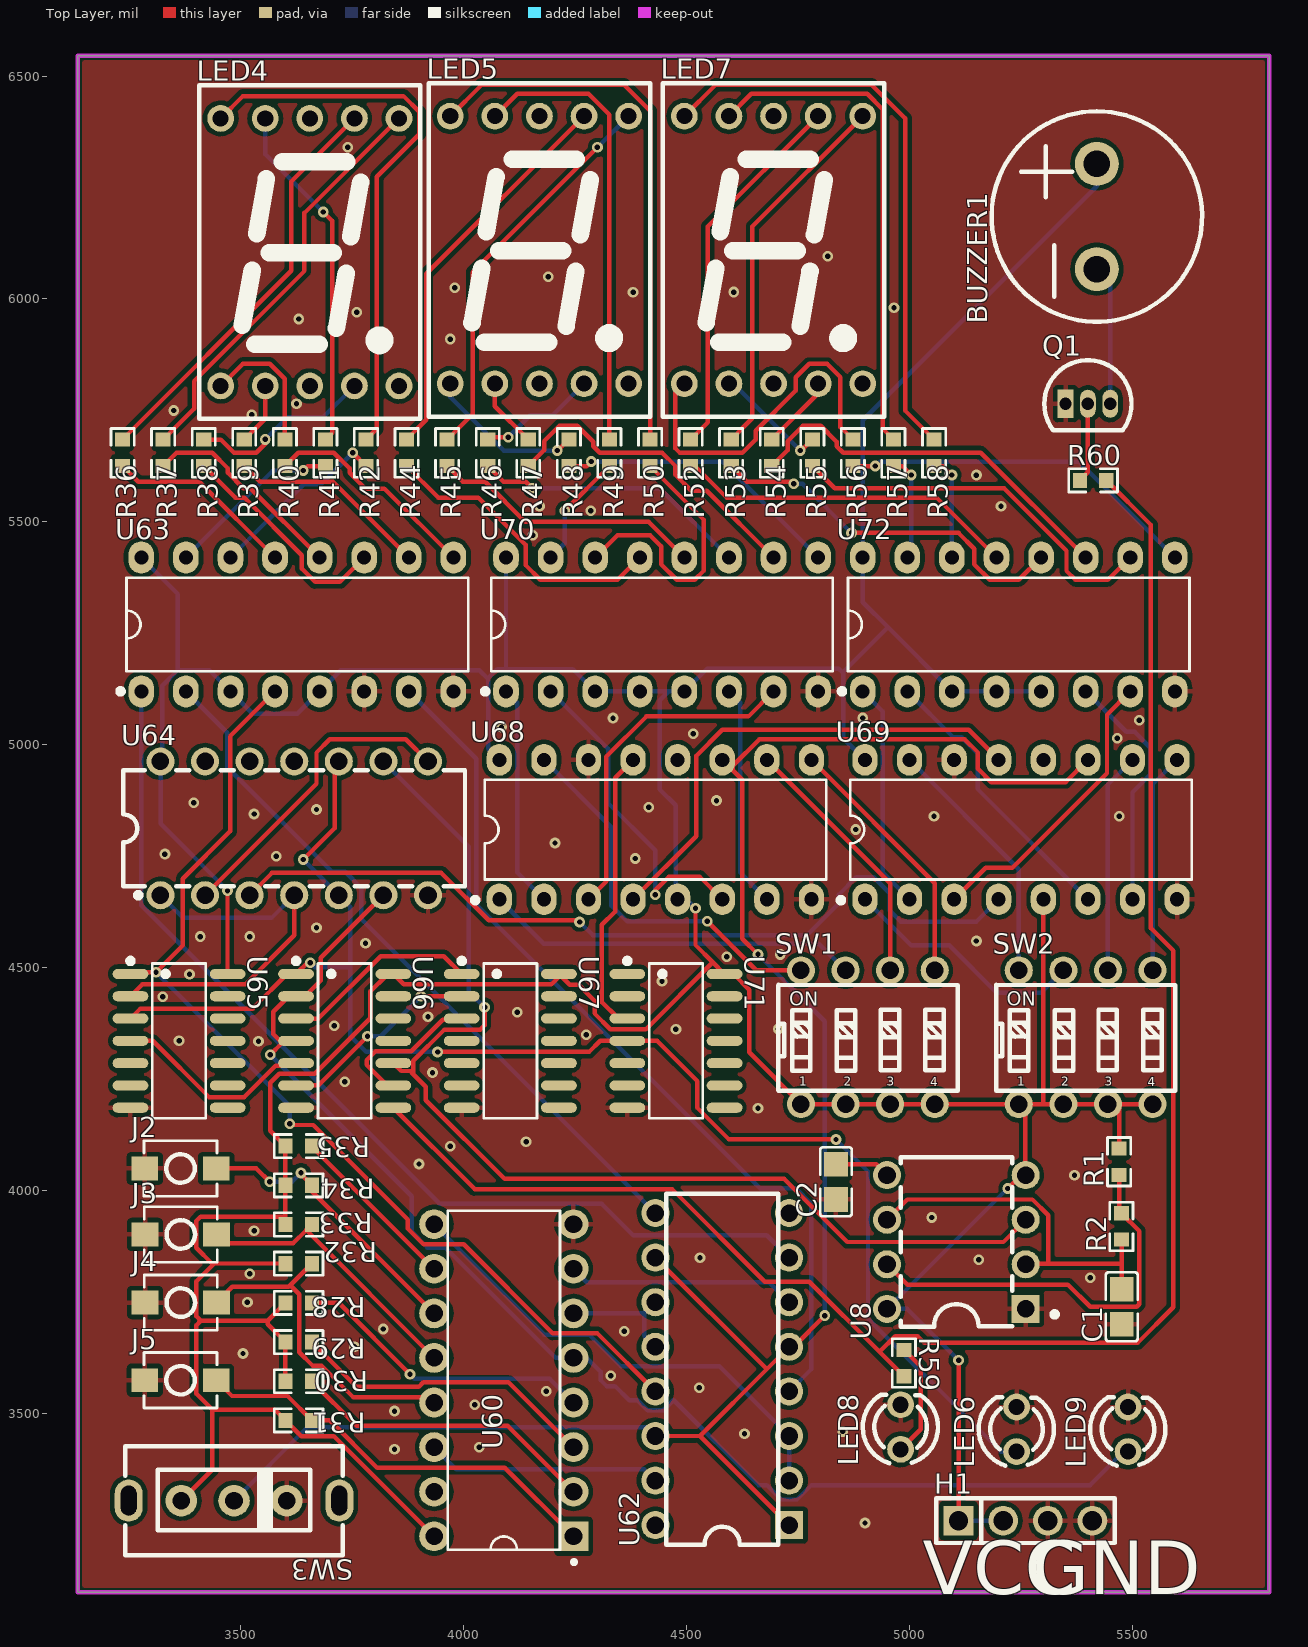
[diagram p0: Top Layer view]
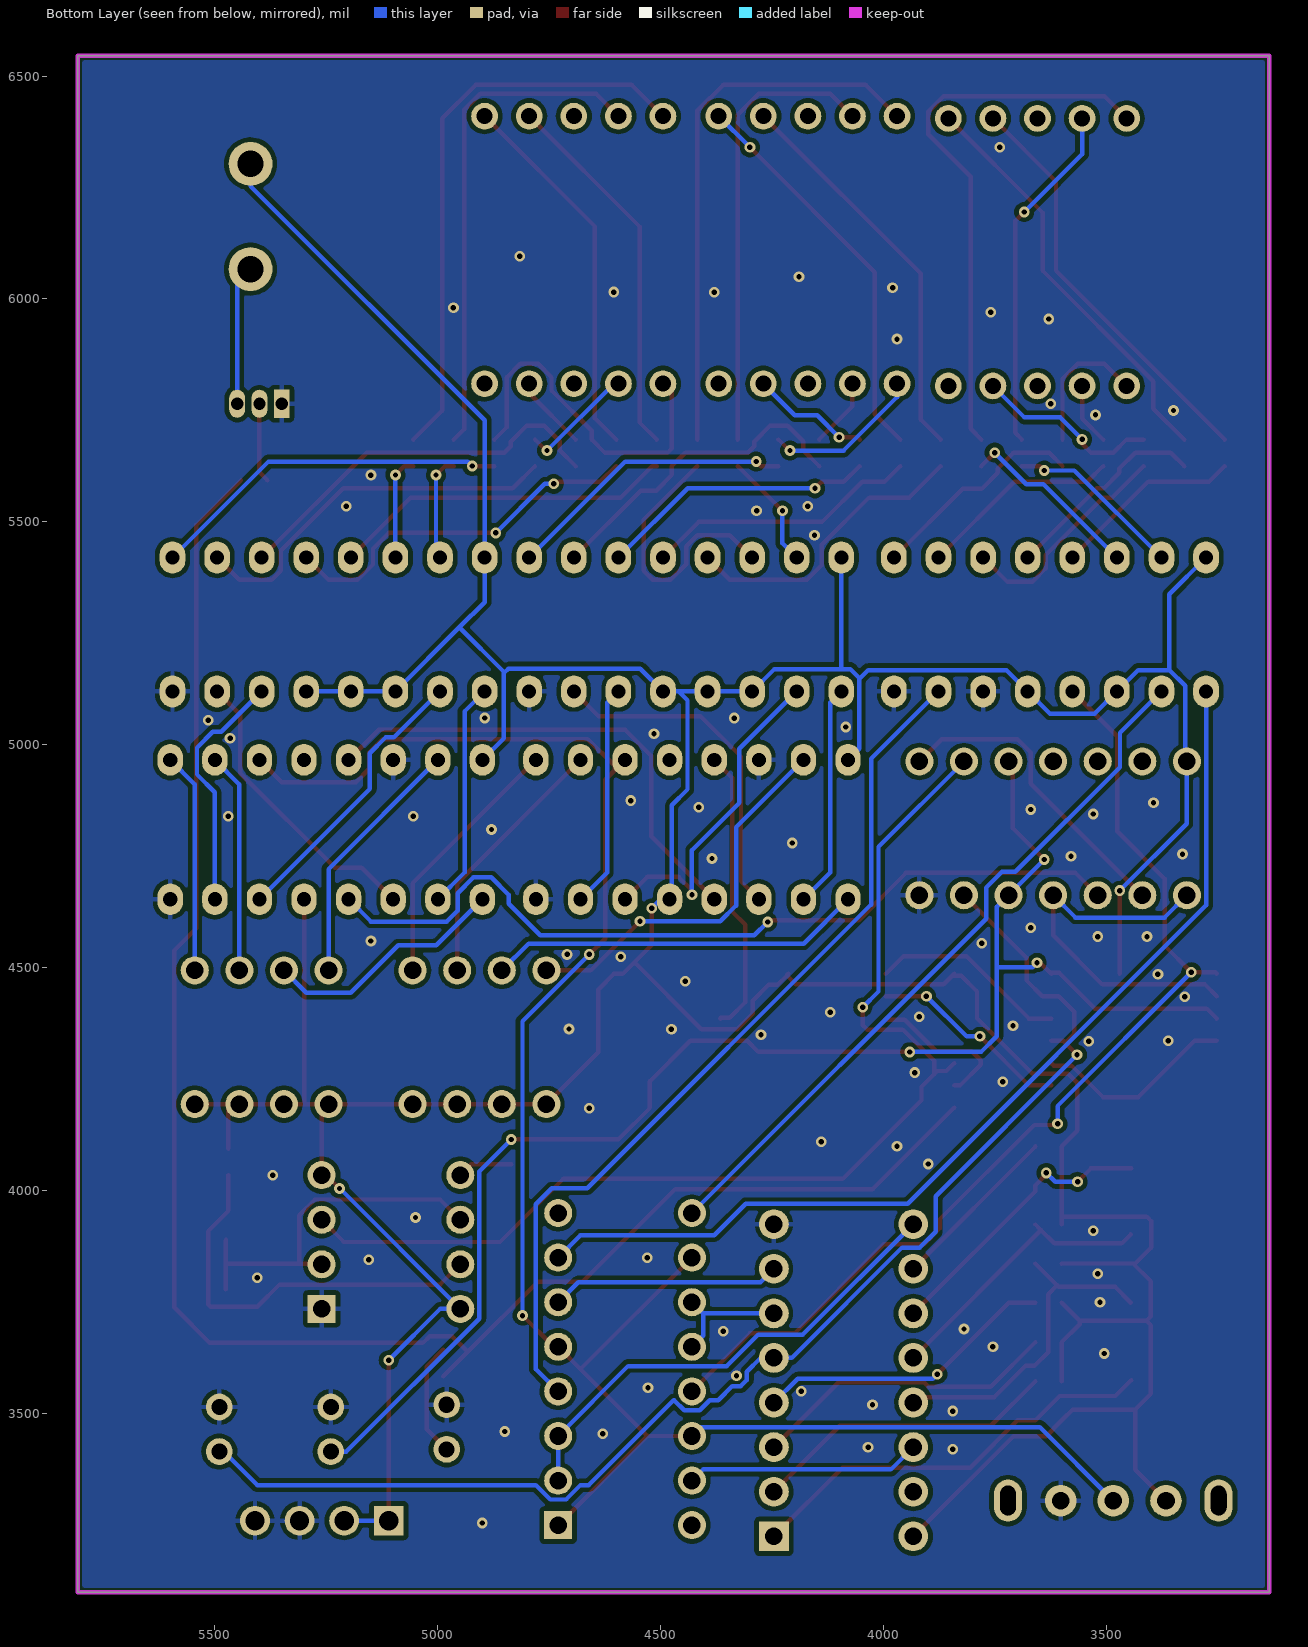
[diagram p1: Bottom Layer view, seen from below]
# Altium PCB MISC75092.pcbdoc
Units mil, origin at the board's own origin, x right, y up, seen from the top; angles counter-clockwise.
Board outline 2672.01 x 3445 mil, 2 copper layers (Top Layer, Bottom Layer), stack 62.206 mil thick; 64 components, 96 nets, 334 pads, 120 vias.

## Layer stack, top to bottom
Top Solder Mask Layer: solder mask 0.394, Dk 3.3
Top Layer: signal copper 1.379
Dielectric1: surface 59.449, FR4, Dk 4.5
Bottom Layer: signal copper 1.378
Bottom Solder Mask Layer: solder mask 0.394, Dk 3.3

## Board outline
3135,6545 3135,3100 5807.01,3100 5807.01,6545

## Design rules (kind name [scope] priority, off if disabled: settings)
BoardOutlineClearance copperThickness2oz_1 [All] p2 off: genericclearance=7.99 ignorepadtopadclearanceinfootprint=FALSE except(0: Arc-SplitContinuation Track-SplitContinuation SMDPad-SplitContinuation THPad-SplitContinuation Via-SplitContinuation Fill-SplitContinuation Region-SplitContinuation Poly-SplitContinuation Text-SplitContinuation Hole-SplitContinuation; 5.98: Arc-CutoutEdge Track-CutoutEdge SMDPad-CutoutEdge THPad-CutoutEdge Via-CutoutEdge Text-CutoutEdge; 6.9: Hole-OutlineEdge Hole-CutoutEdge; 10: Poly-OutlineEdge Poly-CutoutEdge; 11.81: Arc-OutlineEdge Track-OutlineEdge SMDPad-OutlineEdge THPad-OutlineEdge Via-OutlineEdge Fill-OutlineEdge Region-OutlineEdge Text-OutlineEdge Fill-CutoutEdge Region-CutoutEdge)
BoardOutlineClearance Plane_innerPlane_1 [All] p4 off: genericclearance=4.02 ignorepadtopadclearanceinfootprint=FALSE except(0: Arc-SplitContinuation Track-SplitContinuation SMDPad-SplitContinuation THPad-SplitContinuation Via-SplitContinuation Fill-SplitContinuation Region-SplitContinuation Poly-SplitContinuation Text-SplitContinuation Hole-SplitContinuation; 5.98: Arc-CutoutEdge Track-CutoutEdge SMDPad-CutoutEdge THPad-CutoutEdge Via-CutoutEdge Text-CutoutEdge; 6.9: Hole-OutlineEdge Hole-CutoutEdge; 10: Poly-OutlineEdge Poly-CutoutEdge; 11.81: Arc-OutlineEdge Track-OutlineEdge SMDPad-OutlineEdge THPad-OutlineEdge Via-OutlineEdge Fill-OutlineEdge Region-OutlineEdge Text-OutlineEdge Fill-CutoutEdge Region-CutoutEdge)
BoardOutlineClearance Copper_copperRegion_1 [All] p6 off: genericclearance=4.02 ignorepadtopadclearanceinfootprint=FALSE except(0: Arc-SplitContinuation Track-SplitContinuation SMDPad-SplitContinuation THPad-SplitContinuation Via-SplitContinuation Fill-SplitContinuation Region-SplitContinuation Poly-SplitContinuation Text-SplitContinuation Hole-SplitContinuation; 5.98: Arc-CutoutEdge Track-CutoutEdge SMDPad-CutoutEdge THPad-CutoutEdge Via-CutoutEdge Text-CutoutEdge; 6.9: Hole-OutlineEdge Hole-CutoutEdge; 10: Poly-OutlineEdge Poly-CutoutEdge; 11.81: Arc-OutlineEdge Track-OutlineEdge SMDPad-OutlineEdge THPad-OutlineEdge Via-OutlineEdge Fill-OutlineEdge Region-OutlineEdge Text-OutlineEdge Fill-CutoutEdge Region-CutoutEdge)
BoardOutlineClearance copperThickness1oz_1 [All] p8: genericclearance=4.02 ignorepadtopadclearanceinfootprint=FALSE except(0: Arc-SplitContinuation Track-SplitContinuation SMDPad-SplitContinuation THPad-SplitContinuation Via-SplitContinuation Fill-SplitContinuation Region-SplitContinuation Poly-SplitContinuation Text-SplitContinuation Hole-SplitContinuation; 5.98: Arc-CutoutEdge Track-CutoutEdge SMDPad-CutoutEdge THPad-CutoutEdge Via-CutoutEdge Text-CutoutEdge; 6.9: Hole-OutlineEdge Hole-CutoutEdge; 10: Poly-OutlineEdge Poly-CutoutEdge; 11.81: Arc-OutlineEdge Track-OutlineEdge SMDPad-OutlineEdge THPad-OutlineEdge Via-OutlineEdge Fill-OutlineEdge Region-OutlineEdge Text-OutlineEdge Fill-CutoutEdge Region-CutoutEdge)
Clearance copperThickness2oz [All] p1 off: gap=7.99 ignorepadtopadclearanceinfootprint=FALSE except(5.98: SMDPad-Track SMDPad-SMDPad THPad-Track SMDPad-THPad THPad-THPad Track-Via SMDPad-Via THPad-Via Via-Via Fill-SMDPad Region-SMDPad Fill-THPad Region-THPad Fill-Via Region-Via Fill-Fill Fill-Region Region-Region Arc-Track Arc-SMDPad Arc-THPad Arc-Via Fill-Arc Region-Arc Arc-Arc Text-Track SMDPad-Text Text-THPad Text-Via Fill-Text Region-Text Arc-Text Text-Text; 6.9: Hole-Track Hole-SMDPad Hole-THPad Hole-Via Fill-Hole Region-Hole Hole-Arc Hole-Text; 10: Poly-Track Poly-SMDPad Poly-THPad Poly-Via Poly-Fill Poly-Region Poly-Poly Poly-Arc Poly-Text Poly-Hole; 11.81: Fill-Track Region-Track)
Clearance Plane_innerPlane [All] p3 off: gap=4.02 ignorepadtopadclearanceinfootprint=FALSE except(5.98: SMDPad-Track SMDPad-SMDPad THPad-Track SMDPad-THPad THPad-THPad Track-Via SMDPad-Via THPad-Via Via-Via Fill-SMDPad Region-SMDPad Fill-THPad Region-THPad Fill-Via Region-Via Fill-Fill Fill-Region Region-Region Arc-Track Arc-SMDPad Arc-THPad Arc-Via Fill-Arc Region-Arc Arc-Arc Text-Track SMDPad-Text Text-THPad Text-Via Fill-Text Region-Text Arc-Text Text-Text; 6.9: Hole-Track Hole-SMDPad Hole-THPad Hole-Via Fill-Hole Region-Hole Hole-Arc Hole-Text; 10: Poly-Track Poly-SMDPad Poly-THPad Poly-Via Poly-Fill Poly-Region Poly-Poly Poly-Arc Poly-Text Poly-Hole; 11.81: Fill-Track Region-Track)
Clearance Copper_copperRegion [All] p5 off: gap=4.02 ignorepadtopadclearanceinfootprint=FALSE except(5.98: SMDPad-Track SMDPad-SMDPad THPad-Track SMDPad-THPad THPad-THPad Track-Via SMDPad-Via THPad-Via Via-Via Fill-SMDPad Region-SMDPad Fill-THPad Region-THPad Fill-Via Region-Via Fill-Fill Fill-Region Region-Region Arc-Track Arc-SMDPad Arc-THPad Arc-Via Fill-Arc Region-Arc Arc-Arc Text-Track SMDPad-Text Text-THPad Text-Via Fill-Text Region-Text Arc-Text Text-Text; 6.9: Hole-Track Hole-SMDPad Hole-THPad Hole-Via Fill-Hole Region-Hole Hole-Arc Hole-Text; 10: Poly-Track Poly-SMDPad Poly-THPad Poly-Via Poly-Fill Poly-Region Poly-Poly Poly-Arc Poly-Text Poly-Hole; 11.81: Fill-Track Region-Track)
Clearance copperThickness1oz [All] p7: gap=4.02 ignorepadtopadclearanceinfootprint=FALSE except(5.98: SMDPad-Track SMDPad-SMDPad THPad-Track SMDPad-THPad THPad-THPad Track-Via SMDPad-Via THPad-Via Via-Via Fill-SMDPad Region-SMDPad Fill-THPad Region-THPad Fill-Via Region-Via Fill-Fill Fill-Region Region-Region Arc-Track Arc-SMDPad Arc-THPad Arc-Via Fill-Arc Region-Arc Arc-Arc Text-Track SMDPad-Text Text-THPad Text-Via Fill-Text Region-Text Arc-Text Text-Text; 6.9: Hole-Track Hole-SMDPad Hole-THPad Hole-Via Fill-Hole Region-Hole Hole-Arc Hole-Text; 10: Poly-Track Poly-SMDPad Poly-THPad Poly-Via Poly-Fill Poly-Region Poly-Poly Poly-Arc Poly-Text Poly-Hole; 11.81: Fill-Track Region-Track)
DiffPairsRouting differentialPair [All] p1: maxlimit=6 minlimit=6 mostfreqgap=6 toplayer_minwidth=5 toplayer_prefwidth=10 toplayer_maxwidth=100 toplayer_mingap=6 toplayer_prefgap=6 toplayer_maxgap=6 bottomlayer_minwidth=5 bottomlayer_prefwidth=10 bottomlayer_maxwidth=100 bottomlayer_mingap=6 bottomlayer_prefgap=6 bottomlayer_maxgap=6 maxuncoupledlength=10
HoleToHoleClearance otherClearance [All] p1: gap=11.81 allowstackedmicrovias=TRUE
Length netLength [All] p1: minlimit=0 maxlimit=0
PasteMaskExpansion pasteMaskExpansion [All] p1: expansion=0
PlaneConnect innerPlane [All] p1: planeconnectstyle=Relief reliefexpansion=20 reliefentries=4 reliefconductorwidth=10 reliefairgap=10
PolygonConnect copperRegion [All] p1: connectstyle=Relief reliefconductorwidth=10 reliefentries=4 polygonreliefangle="90 Angle" airgapwidth=10 via.connectstyle=Relief via.reliefconductorwidth=10 via.reliefentries=4 via.polygonreliefangle="90 Angle" via.airgapwidth=10
RoutingVias viaSize [All] p1: holewidth=12.01 width=24.02 viastyle="Through Hole" minholewidth=11.81 minwidth=19.68 maxholewidth=248.03 maxwidth=393.7
SolderMaskExpansion solderMaskExpansion [IsVia] p1: expansion=-1000 istentingtop=TRUE
SolderMaskExpansion solderMaskExpansion [All] p2: expansion=2 istentingtop=FALSE
Width copperThickness2oz_2 [All] p1 off: maxlimit=100 minlimit=8 preferedwidth=10
Width copperThickness1oz_2 [All] p2: maxlimit=100 minlimit=5 preferedwidth=10

## Components (designator, comment, footprint, x,y, rotation, side; value= is the part's Value field where it differs from the comment)
BUZZER1 "buzzer" BUZ-TH_BD12.0-P6.00-D0.9-RD 5420,6185 r90 top
C1 "100uF" C0805 5475.94,3739.74 r90 top
C2 "10nF" C0805 4835,4020 r90 top
H1 "" HDR-TH_4P-P2.54-V-M 5260,3260 r0 top
J2 "Tact switch 3*4*H" SW-SMD_L4.0-W2.9-LS5.0 3365,4050 r0 top
J3 "Tact switch 3*4*H" SW-SMD_L4.0-W2.9-LS5.0 3365.61,3902.01 r0 top
J4 "Tact switch 3*4*H" SW-SMD_L4.0-W2.9-LS5.0 3365.61,3749.1 r0 top
J5 "Tact switch 3*4*H" SW-SMD_L4.0-W2.9-LS5.0 3365,3575 r0 top
LED4 "" LED-SEG-TH_10P-L12.6-W19.0-P2.54-S15.24-BL 3655,6105 r0 top
LED5 "" LED-SEG-TH_10P-L12.6-W19.0-P2.54-S15.24-BL 4170,6110 r0 top
LED6 "" LED_TH-3mm 5240,3465 r90 top
LED7 "" LED-SEG-TH_10P-L12.6-W19.0-P2.54-S15.24-BL 4695,6110 r0 top
LED8 "" LED_TH-3mm 4980,3470 r90 top
LED9 "" LED_TH-3mm 5490,3465 r90 top
Q1 "2N2222A" TO-92-3_L4.9-W3.7-P1.27-L 5400,5765 r0 top
R1 "10k" R0603 5470,4065 r90 top
R2 "2.2k" R0603 5475,3920 r90 top
R28 "10k" R0603 3630,3748.57 r180 top
R29 "10k" R0603 3630,3660.71 r180 top
R30 "10k" R0603 3630,3572.86 r180 top
R31 "10k" R0603 3630,3485 r180 top
R32 "10k" R0603 3630,3836.43 r180 top
R33 "10k" R0603 3630,3924.29 r180 top
R34 "10k" R0603 3630,4012.14 r180 top
R35 "10k" R0603 3630,4100 r180 top
R36 "330" R0603 3235,5655 r90 top
R37 "330" R0603 3326,5655 r90 top
R38 "330" R0603 3417,5655 r90 top
R39 "330" R0603 3508,5655 r90 top
R40 "330" R0603 3599,5655 r90 top
R41 "330" R0603 3690,5655 r90 top
R42 "330" R0603 3781,5655 r90 top
R44 "330" R0603 3872,5655 r90 top
R45 "330" R0603 3963,5655 r90 top
R46 "330" R0603 4054,5655 r90 top
R47 "330" R0603 4145,5655 r90 top
R48 "330" R0603 4236,5655 r90 top
R49 "330" R0603 4327,5655 r90 top
R50 "330" R0603 4418,5655 r90 top
R52 "330" R0603 4509,5655 r90 top
R53 "330" R0603 4600,5655 r90 top
R54 "330" R0603 4691,5655 r90 top
R55 "330" R0603 4782,5655 r90 top
R56 "330" R0603 4873,5655 r90 top
R57 "330" R0603 4964,5655 r90 top
R58 "330" R0603 5055,5655 r90 top
R59 "500" R0603 4987.46,3613.5 r270 top
R60 "2k" R0603 5411.68,5593.17 r0 top
SW1 "DIP switch EI-04" SW-TH_DIPSWITCHEI-04 4906.51,4344.24 r0 top
SW2 "DIP switch EI-04" SW-TH_DIPSWITCHEI-04 5395,4344.24 r0 top
SW3 "SWITCH-slide three-pin two-position" SW-TH_C9900003112 3485,3305 r180 top
U8 "NE555PE4" PDIP-8_L9.6-W6.4-P2.54-LS7.9-BL-1 5105,3885 r90 top
U60 "SN74148N" PDIP-16_L19.3-W6.4-P2.54-LS7.9-BL 4090,3575 r90 top
U62 "74279N" DIP-16_L19.8-W6.5-P2.54-LS7.6-BL 4580,3600 r90 top
U63 "SN74LS48N" DIP-16_L19.3-W6.4-P2.54-LS7.6-BL 3627.01,5270 r0 top
U64 "SN74LS00N(LX)" PDIP-14_L19.3-W6.4-P2.54-LS7.9-BL 3620,4812.75 r0 top
U65 "SN74LS04DR" SOIC-14_L8.7-W3.9-P1.27-LS6.0-BL 3361.8,4336.18 r270 top
U66 "SN74LS08DR(LX)" SOIC-14_L8.7-W3.9-P1.27-LS6.0-BL 3733.22,4336.18 r270 top
U67 "SN74LS32DR" SOIC-14_L8.7-W3.9-P1.27-LS6.0-BL 4104.64,4336.18 r270 top
U68 "SN74LS192N(LX)" PDIP-16_L19.3-W6.4-P2.54-LS7.94-BL 4430,4810 r0 top
U69 "SN74LS192N(LX)" PDIP-16_L19.3-W6.4-P2.54-LS7.94-BL 5250,4810 r0 top
U70 "SN74LS48N" DIP-16_L19.3-W6.4-P2.54-LS7.6-BL 4445,5270 r0 top
U71 "SN74LS04DR" SOIC-14_L8.7-W3.9-P1.27-LS6.0-BL 4476.06,4336.18 r270 top
U72 "SN74LS48N" DIP-16_L19.3-W6.4-P2.54-LS7.6-BL 5245,5270 r0 top

## Footprints (in the part's own frame and the unit in brackets; to place one, negate y for a bottom-side part, rotate by r counter-clockwise, add the part's x,y. Pads: shape width x height; smd on the part's side, far side on the other; paste and mask are expansions set on the pad)
BUZ-TH_BD12.0-P6.00-D0.9-RD [mm]
  round 2.5 hole 1.5 paste+0 mask+0.05: 1(-3,0) 2(3,0)
  silkscreen extent -5.99,-5.99 5.99,5.99
C0805 [mm]
  rect 1.41x1.35 smd paste-100 mask+0.051: 1(-1,0) 2(1,0)
  silkscreen extent -1.96,-0.9 1.96,0.9
DIP-16_L19.3-W6.4-P2.54-LS7.6-BL [mm]
  oval 1.46x1.825 hole 0.8: 1(-8.89,-3.81) 2(-6.35,-3.81) 3(-3.81,-3.81) 4(-1.27,-3.81) 5(1.27,-3.81) 6(3.81,-3.81) 7(6.35,-3.81) 8(8.89,-3.81) 9(8.89,3.81) 10(6.35,3.81) 11(3.81,3.81) 12(1.27,3.81) 13(-1.27,3.81) 14(-3.81,3.81) 15(-6.35,3.81) 16(-8.89,3.81)
  silkscreen extent -10.22,-3.96 9.73,2.67
DIP-16_L19.8-W6.5-P2.54-LS7.6-BL [mm]
  rect 1.6x1.6 hole 1: 1(-8.89,-3.81)
  round 1.6 hole 1 copper offset 0,0: 2(-6.35,-3.81) 3(-3.81,-3.81) 4(-1.27,-3.81) 5(1.27,-3.81) 6(3.81,-3.81) 7(6.35,-3.81) 8(8.89,-3.81) 9(8.89,3.81) 10(6.35,3.81) 11(3.81,3.81) 12(1.27,3.81) 13(-1.27,3.81) 14(-3.81,3.81) 15(-6.35,3.81) 16(-8.89,3.81)
  silkscreen extent -10,-3.2 10,3.2
HDR-TH_4P-P2.54-V-M [mm]
  rect 1.7x1.7 hole 1.1: 1(-3.81,0)
  round 1.7 hole 1.1: 2(-1.27,0) 3(1.27,0) 4(3.81,0)
  silkscreen extent -5.08,-1.27 5.08,1.27
LED-SEG-TH_10P-L12.6-W19.0-P2.54-S15.24-BL [mil]
  round 60 hole 36: 1(-200,-300) 2(-100,-300) 3(0,-300) 4(100,-300) 5(200,-300) 6(200,300) 7(100,300) 8(0,300) 9(-100,300) 10(-200,300)
  silkscreen extent -248,-374 248,374
LED_TH-3mm [mil]
  round 60 hole 36 paste+0 mask+2: 1(-50,0) 2(50,0)
  silkscreen extent -81,-84 72,85
PDIP-8_L9.6-W6.4-P2.54-LS7.9-BL-1 [mil]
  rect 63x63 hole 39.37: 1(-150,-155.51)
  round 63 hole 39.37: 2(-50,-155.51) 3(50,-155.51) 4(150,-155.51) 5(150,155.52) 6(50,155.52) 7(-50,155.52) 8(-150,155.52)
  silkscreen extent -190,-226 190,125
PDIP-14_L19.3-W6.4-P2.54-LS7.9-BL [mm]
  round 1.6 hole 1: 1(-7.62,-3.81) 2(-5.08,-3.81) 3(-2.54,-3.81) 4(0,-3.81) 5(2.54,-3.81) 6(5.08,-3.81) 7(7.62,-3.81) 8(7.62,3.81) 9(5.08,3.81) 10(2.54,3.81) 11(0,3.81) 12(-2.54,3.81) 13(-5.08,3.81) 14(-7.62,3.81)
  silkscreen extent -9.73,-3.96 9.73,3.3
PDIP-16_L19.3-W6.4-P2.54-LS7.9-BL [mm]
  rect 1.7x1.7 hole 1: 1(-8.89,-3.97)
  round 1.7 hole 1 copper offset 0,0: 2(-6.35,-3.97) 3(-3.81,-3.97) 4(-1.27,-3.97) 5(1.27,-3.97) 6(3.81,-3.97) 7(6.35,-3.97) 8(8.89,-3.97)
  round 1.7 hole 1: 9(8.89,3.97) 10(6.35,3.97) 11(3.81,3.97) 12(1.27,3.97) 13(-1.27,3.97) 14(-3.81,3.97) 15(-6.35,3.97) 16(-8.89,3.97)
  silkscreen extent -10.46,-4.1 9.65,3.2
PDIP-16_L19.3-W6.4-P2.54-LS7.94-BL [mm]
  oval 1.44x1.8 hole 0.8: 1(-8.89,-3.97) 2(-6.35,-3.97) 3(-3.81,-3.97) 4(-1.27,-3.97) 5(1.27,-3.97) 6(3.81,-3.97) 7(6.35,-3.97) 8(8.89,-3.97) 9(8.89,3.97) 10(6.35,3.97) 11(3.81,3.97) 12(1.27,3.97) 13(-1.27,3.97) 14(-3.81,3.97) 15(-6.35,3.97) 16(-8.89,3.97)
  silkscreen extent -10.41,-4.17 9.73,2.84
R0603 [mil]
  rect 31.75x34.02 smd paste-3937.01 mask+2: 1(-29.66,0) 2(29.66,0)
  silkscreen extent -55,-26 55,26
SOIC-14_L8.7-W3.9-P1.27-LS6.0-BL [mil]
  oval 22.6x80.24 smd: 1(-150,-109.02) 2(-100,-109.02) 3(-50,-109.02) 4(0,-109.02) 5(50,-109.02) 6(100,-109.02) 7(150,-109.02) 8(150,109.02) 9(100,109.02) 10(50,109.02) 11(0,109.02) 12(-50,109.02) 13(-100,109.02) 14(-150,109.02)
  silkscreen extent -185,-115 173,60
SW-SMD_L4.0-W2.9-LS5.0 [mm]
  rect 1.53x1.36 smd: 1(-2.035,0) 2(2.035,0)
  silkscreen extent -2.08,-1.58 2.08,1.58
SW-TH_C9900003112 [mm]
  round 1.8 hole 1: 1(-3,0) 2(0,0) 3(3,0)
  oval 1.6x2.4 hole 0.9 slot 1.7 at 90 deg: EH(-6,0) EH(6,0)
  silkscreen extent -6.2,-3.1 6.2,3.1
SW-TH_DIPSWITCHEI-04 [mm]
  round 1.6 hole 1: 1(-3.81,-3.81) 2(-1.27,-3.81) 3(1.27,-3.81) 4(3.81,-3.81) 5(3.81,3.81) 6(1.27,3.81) 7(-1.27,3.81) 8(-3.81,3.81)
  silkscreen extent -5.1,-3.05 5.11,2.98
TO-92-3_L4.9-W3.7-P1.27-L [mm]
  rect 0.9x1.6 hole 0.7: 1(-1.27,0)
  oval 0.9x1.6 hole 0.7: 2(0,0) 3(1.27,0)
  silkscreen extent -2.48,-1.5 2.48,2.48

## Via types
v1: diameter 24.02, hole 12, Top Layer to Bottom Layer, 119 vias
v2: diameter 24, hole 12, Top Layer to Bottom Layer, 1 vias

## Nets (pads, with @x,y where several pads share a name; then routed paths per layer and width w, separated by ;. In a path a pad name is that pad's centre, name@x,y a point inside that pad or via, vN(x,y) a via of type N, cw(c..) or ccw(c..) an arc to the next point about the centre after c; other vN are vias at no path point)
$1N419: R1.1 R2.2 U8.7 | length 915.9
  Top Layer w10: U8.7 4994.83,3789.66 5355,3789.66 5405,3739.66 5509.24,3739.66 5515,3745.42 5515,3909.66 R2.2 5470,3954.66 R1.1
$1N420: C1.2 R2.1 U8.2 U8.6 | length 831
  Top Layer w10: U8.6 4994.85,3980.36 5275.58,3980.36 5310.94,3945 5310.94,3836.61 ; U8.2 5262.12,3836.61 5310.94,3836.61 ; R2.1 5475.94,3889.4 5475.94,3836.61 ; C1.2 5475.94,3836.61 ; 5310.94,3836.61 5475.94,3836.61
$1N421: C2.2 U8.5 | length 124.6
  Top Layer w10: C2.2 4925.12,4059.37 U8.5
$1N5737: J3.2 R33.1 U60.12 | length 645.4
  Top Layer w10: J3.2 3465.73,3882.01 3617.39,3882.01 R33.1@3647.44,3912.06 ; R33.1 R33.1@3647.44,3912.06 ; U60.12 3647.44,3911.26 R33.1@3647.44,3912.06
$1N8555: R35.1 U60.10 | length 388.5
  Top Layer w10: R35.1 3659.66,4099.04 U60.10
$1N8560: J2.2 R34.1 U60.11 | length 649.4
  Top Layer w10: J2.2 3535.12,4050 v1(3565.12,4020) ; v1(3635.12,4040) 3635.12,4036.68 R34.1 3659.66,3999.04 U60.11
  Bottom Layer w10: v1(3565.12,4020) 3615.12,4020 v1(3635.12,4040)
$1N8572: J4.2 R32.1 U60.13 | length 757.7
  Top Layer w10: J4.2 3481.08,3784.45 3607.68,3784.45 3611.22,3787.99 ; R32.1 3611.22,3787.99 ; U60.13 3921.42,3537.28 3751.93,3537.28 3681.22,3607.99 3661.22,3607.99 3631.22,3637.99 3631.22,3767.99 3611.22,3787.99
$1N8578: J5.2 R31.1 U60.1 | length 946.2
  Top Layer w10: J5.2 3480.48,3539.64 3605.02,3539.64 R31.1 3699.66,3485 3805.73,3378.93 4092.37,3378.93 U60.1
$1N8584: R30.1 U60.2 | length 689.3
  Top Layer w10: R30.1 3759.66,3472.86 4098.44,3472.86 U60.2
$1N8590: R29.1 U60.3 | length 692.6
  Top Layer w10: R29.1 3759.66,3560.71 3899.66,3560.71 3909.66,3570.71 4100.59,3570.71 U60.3
$1N8596: R28.1 U60.4 | length 679.2
  Top Layer w10: R28.1 3719.66,3748.57 v1(3879.66,3588.57)
  Bottom Layer w10: v1(3879.66,3588.57) 3889.66,3578.57 4192.73,3578.57 U60.4
$1N11433: U60.9 U62.2 U62.3 | length 1093.1
  Bottom Layer w10: U60.9 4181.19,3677.51 4281.19,3677.51 4351.9,3606.8 4573.2,3606.8 U62.3 U62.2
$1N11448: U60.7 U62.6 | length 514.8
  Bottom Layer w10: U60.7 4276.3,3795 4685,3795 U62.6
$1N11455: U60.6 U62.11 U62.12 | length 279.4
  Bottom Layer w10: U60.6 4405,3725 ; U62.12 4405,3675 4405,3725 ; U62.11 4405,3725
$1N11473: U60.14 U62.15 | length 527.4
  Bottom Layer w10: U60.14 3983.7,3375 4405,3375 U62.15
$1N11481: SW3.2 U62.1 U62.5 U62.10 U62.14 U68.11 U69.11 | length 4406.2
  Top Layer w10: U62.14 4530,3450 4531.77,3451.77 ; U62.10 4679.74,3600.26 4680.26,3600.26 ; U68.11 4603.43,4942.87 ; v1(4660,4530) 4624.64,4565.36 4624.64,4921.66 4603.43,4942.87 ; U62.1 4531.77,3448.23 4531.77,3451.77 ; v1(4810,3720) 4740,3650 U62.5 4680.26,3600.26 ; U69.11 5350,4916.3 5183.43,4916.3 5153.43,4946.3 5153.43,4982.87 5123.43,5012.87 4663.43,5012.87 4603.43,4952.87 4603.43,4942.87 ; 4531.77,3451.77 4680.26,3600.26
  Bottom Layer w10: SW3.2 3650,3470 4410,3470 U62.14 ; v1(4660,4530) 4810,4380 v1(4810,3720)
$1N11844: LED4.7 R36.2 | length 935.7
  Top Layer w10: R36.2 3613.58,6063.24 3613.58,6263.58 LED4.7
$1N11846: LED4.6 R37.2 | length 939.5
  Top Layer w10: R37.2 3395.38,5754.04 3395.38,5815.38 3642.87,6062.87 3642.87,6192.87 LED4.6
$1N11848: LED4.4 R38.2 | length 418.3
  Top Layer w10: R38.2 3455.34,5684.66 3485,5655 3535,5655 3555,5675 v1(3555,5685)
  Bottom Layer w10: v1(3555,5685) 3604.29,5734.29 3684.29,5734.29 LED4.4
$1N11850: LED4.2 R39.2 | length 139.8
  Top Layer w10: R39.2 3555,5731.66 LED4.2
$1N11852: LED4.1 R40.2 | length 315.1
  Top Layer w10: LED4.1 3505,5855 3565,5855 3599,5821 R40.2
$1N11854: LED4.9 R41.2 | length 788.7
  Top Layer w10: v1(3685,6195) 3705,6175 3705,5699.66 R41.2
  Bottom Layer w10: LED4.9 3555,6325 v1(3685,6195)
$1N11856: LED4.10 R42.2 | length 1265.1
  Top Layer w10: LED4.10 3505,6455 3865,6455 3900.36,6419.64 3900.36,6369.64 3805,6274.29 3805,5708.66 R42.2
$1N14663: R36.1 U63.13 | length 427.1
  Top Layer w10: R36.1 3270.36,5589.98 3407.03,5589.98 U63.13
$1N14665: R37.1 U63.12 | length 466.8
  Top Layer w10: R37.1 3356,5655.34 3436,5655.34 3471.36,5619.98 3471.36,5609.98 3506,5575.34 3521.67,5575.34 U63.12
$1N14667: R38.1 U63.11 | length 507.9
  Top Layer w10: R38.1 3487.71,5554.63 3507.71,5554.63 3637,5425.34 3637,5395.34 3667,5365.34 3722.35,5365.34 U63.11
$1N14669: R39.1 U63.10 | length 454.1
  Top Layer w10: R39.1 3543.36,5589.98 3707.03,5589.98 U63.10
$1N14671: R40.1 U63.9 | length 493.8
  Top Layer w10: R40.1 3629,5655.34 3709,5655.34 3744.36,5619.98 3744.36,5609.98 3779.71,5574.63 3822.38,5574.63 U63.9
$1N14673: R41.1 U63.15 | length 398
  Top Layer w10: v1(3640,5615.34) 3650,5625.34 R41.1
  Bottom Layer w10: U63.15 3572.35,5615.34 v1(3640,5615.34)
$1N14675: R42.1 U63.14 | length 413.9
  Top Layer w10: v1(3751,5655.34) R42.1
  Bottom Layer w10: U63.14 3641.64,5584.63 3680.29,5584.63 v1(3751,5655.34)
$1N14679: U62.4 U63.7 | length 2011.6
  Bottom Layer w10: U63.7 4028.25,4968.77 4028.25,4641.75 4664.64,4005.36 4744.64,4005.36 4780,3970 4780,3600 U62.4
$1N14684: U62.7 U63.1 | length 2260.2
  Bottom Layer w10: U63.1 3277.01,4640 3946.3,3970.71 4309.29,3970.71 4380,3900 4680,3900 U62.7
$1N14690: U62.9 U63.2 | length 1623.7
  Bottom Layer w10: U63.2 3470,5027.01 3470,4950 3704.64,4715.36 3734.64,4715.36 3770,4680 3770,4610 U62.9
$1N32087: U66.3 U67.1 | length 446
  Top Layer w10: U66.3 3674.2,4386.18 3814.2,4526.18 3955.62,4526.18 U67.1
$1N32091: U66.6 U67.2 | length 454.3
  Top Layer w10: U66.6 3674.2,4236.18 v1(3784.2,4346.18) ; v1(3904.2,4436.18) U67.2
  Bottom Layer w10: v1(3784.2,4346.18) 3814.2,4346.18 v1(3904.2,4436.18)
$1N32097: LED9.1 U60.5 U64.6 U66.2 U66.4 | length 2992.1
  Top Layer w10: v1(3566.3,4305) U66.4@3592.82,4331.52 ; U66.4 3597.48,4336.18 U66.4@3592.82,4331.52 ; U64.6 3679.55,4522.31 3679.55,4471.54 3644.2,4436.18 U66.2 3607.48,4436.18 3572.82,4401.52 3572.82,4351.52 U66.4@3592.82,4331.52
  Bottom Layer w10: v1(3566.3,4305) 3883.46,3987.84 3883.46,3907.84 3918.81,3872.49 3958.81,3872.49 4206.3,3625 U60.5 4276.3,3625 4307.01,3594.29 4307.01,3575.48 4320.48,3562.01 4339.29,3562.01 4371.3,3530 4389.92,3530 4412.4,3507.52 4447.6,3507.52 4470.08,3530 4471.3,3530 4661.3,3340 4679.92,3340 4712.4,3307.52 4747.6,3307.52 4780.08,3340 5405,3340 5480,3415 LED9.1
$1N32112: U65.4 U66.5 | length 455.1
  Top Layer w10: U65.4 3302.78,4336.18 3428.85,4210.12 3508.13,4210.12 3578.84,4280.83 3618.84,4280.83 U66.5
$1N32117: LED6.1 U64.5 U64.10 U65.3 U66.1 U71.4 | length 3375
  Top Layer w10: U65.3 3275.19,4408.6 3526.61,4408.6 3606.61,4488.6 U66.1@3626.61,4488.6 ; U66.1 U66.1@3626.61,4488.6 ; v1(3640,4742.75) 3710.71,4813.46 3710.71,4953.46 U64.10 ; v1(3656.18,4511.58) 3649.59,4511.58 U66.1@3626.61,4488.6 ; v1(3941.53,4311.22) 4281.22,4311.22 4306.18,4336.18 4433.82,4336.18 4524.29,4245.71 4524.29,4185.71 4595,4115 v1(4835,4115)
  Bottom Layer w10: v1(3640,4742.75) U64.5 3746.18,4636.58 3746.18,4501.58 ; v1(3656.18,4511.58) 3666.18,4501.58 3746.18,4501.58 ; v1(3941.53,4311.22) 3781.53,4311.22 3746.18,4346.58 3746.18,4501.58 ; v1(4835,4115) 4906.8,4043.2 4906.8,3713.2 5205,3415 LED6.1
$1N32139: U64.2 U64.8 | length 706.7
  Top Layer w10: U64.2 3670,4912.75 3670,4982.75 3700,5012.75 3870,5012.75 U64.8
$1N32157: U8.3 U64.9 U66.10 | length 2531.1
  Top Layer w10: U66.10 3859.87,4268.55 3879.87,4268.55 3886.94,4261.48 ; v1(4046.94,4411.48) 4046.94,4371.48 4036.94,4361.48 3956.94,4361.48 3886.94,4291.48 3886.94,4261.48 ; U8.3 5210.51,3885 4860.51,3885 4719.09,4026.42 4092,4026.42 3915.22,4203.2 3915.22,4233.2 3886.94,4261.48
  Bottom Layer w10: U64.9 4011.58,4771.17 4011.58,4446.84 v1(4046.94,4411.48)
$1N32178: U66.9 U67.3 | length 341.4
  Top Layer w10: U66.9 3828.86,4236.18 3782.24,4282.81 3782.24,4292.81 3802.24,4312.81 3882.24,4312.81 3952.95,4383.52 3992.95,4383.52 U67.3
$1N32232: U64.1 U64.4 U65.2 | length 855.2
  Top Layer w10: U65.2 3279.35,4462.75 3510,4462.75 3620,4572.75 U64.4
  Bottom Layer w10: U64.1 3370,4612.75 3570,4612.75 U64.4
$1N32241: U62.13 U63.4 U65.1 | length 2343.9
  Top Layer w10: U65.1 3256.6,4490 v1(3310,4490) 3370,4550 3370,4700 3476.07,4806.07 3476.07,5019.05 U63.4 ; v1(3610,4150) 3612.51,4147.49 3662.51,4147.49 3874.64,3935.36 3874.64,3915.36 3910,3880 4000,3880 4200,3680 4300,3680 U62.13
  Bottom Layer w10: v1(3310,4490) 3610,4190 v1(3610,4150)
$1N38590: LED5.7 R44.2 | length 890.2
  Top Layer w10: R44.2 3916.45,5729.11 3916.45,6056.45 LED5.7
$1N38591: LED5.6 R45.2 | length 893.9
  Top Layer w10: R45.2 4020,5741.66 4020,6060 v1(4300,6340)
  Bottom Layer w10: v1(4300,6340) LED5.6
$1N38592: LED5.4 R46.2 | length 267.9
  Top Layer w10: R46.2 4059.34,5690 v1(4100,5690)
  Bottom Layer w10: v1(4100,5690) 4149.29,5739.29 4199.29,5739.29 LED5.4
$1N38593: LED5.2 R47.2 | length 156.4
  Top Layer w10: LED5.2 4070,5759.66 R47.2
$1N38594: LED5.1 R48.2 | length 355.9
  Top Layer w10: v1(4210,5660) 4211.34,5660 R48.2
  Bottom Layer w10: LED5.1 3970,5780 4090,5660 v1(4210,5660)
$1N38595: LED5.9 R49.2 | length 1025.5
  Top Layer w10: LED5.9 4120,6460 4280,6460 4327,6413 R49.2
$1N38596: LED5.10 R50.2 | length 1238.4
  Top Layer w10: LED5.10 4040,6480 4360,6480 4418,6422 R50.2
$1N38598: R44.1 U70.13 | length 676
  Top Layer w10: R44.1 3942.71,5554.63 4032.71,5554.63 4138.78,5448.56 4138.78,5403.22 4172,5370 4345,5370 U70.13
$1N38599: R45.1 U70.12 | length 617.1
  Top Layer w10: R45.1 3998.36,5589.98 4048.36,5589.98 4138.36,5499.98 4415.02,5499.98 U70.12
$1N38600: R46.1 U70.11 | length 626.1
  Top Layer w10: R46.1 4089.36,5589.98 4139.36,5589.98 v1(4154,5575.34)
  Bottom Layer w10: v1(4154,5575.34) 4439.66,5575.34 U70.11
$1N38601: R47.1 U70.10 | length 738.9
  Top Layer w10: R47.1 4180.36,5660.7 4180.36,5680.7 4215,5715.34 4255,5715.34 4290.36,5679.98 4290.36,5669.98 4305,5655.34 4445,5655.34 4475,5625.34 4475,5605.34 4510.36,5569.98 4545.02,5569.98 U70.10
$1N38602: R48.1 U70.9 | length 652.3
  Top Layer w10: R48.1 4276,5625.34 v1(4286,5635.34)
  Bottom Layer w10: v1(4286,5635.34) 4579.66,5635.34 U70.9
$1N38603: R49.1 U70.15 | length 260
  Top Layer w10: v1(4227,5525.34) R49.1
  Bottom Layer w10: U70.15 4227,5452 v1(4227,5525.34)
$1N38604: R50.1 U70.14 | length 621.9
  Top Layer w10: U70.14 4345,5470 4418,5470 4442.64,5445.36 4442.64,5405.36 4478,5370 4518,5370 4538,5390 4538,5505.34 R50.1
$1N38628: U68.3 U70.7 | length 772.2
  Top Layer w10: U68.3 4320,4693.7 4320,4973.7 4410,5063.7 4638.7,5063.7 U70.7
$1N38636: U68.2 U70.1 | length 501.5
  Bottom Layer w10: U70.1 4120,5095 4120,4713.7 U68.2
$1N38644: U68.6 U70.2 | length 746.8
  Top Layer w10: v1(4430,4663.7) 4430,4673.7 4460,4703.7 4530,4703.7 U68.6
  Bottom Layer w10: U70.2 4323.93,4991.07 4323.93,4869.77 4430,4763.7 v1(4430,4663.7)
$1N38648: U68.7 U70.6 | length 501.5
  Bottom Layer w10: U70.6 4620,5095 4620,4713.7 U68.7
$1N38743: U68.13 U71.3 | length 644.5
  Top Layer w10: U71.3 4365.36,4387.86 4345.36,4387.86 4310,4423.22 4310,4596.3 4340,4626.3 4340,4926.3 U68.13
$1N38887: SW1.7 U68.1 | length 842.6
  Bottom Layer w10: U68.1 4179.46,4554.24 4796.51,4554.24 SW1.7
$1N38889: SW1.5 U68.9 | length 586.6
  Top Layer w10: U68.9 5056.51,4689.79 SW1.5
$1N38891: SW1.6 U68.10 | length 586.6
  Top Layer w10: U68.10 4956.51,4689.79 SW1.6
$1N38893: SW1.8 U68.15 | length 874.9
  Top Layer w10: v1(4546.51,4604.24) 4656.51,4494.24 SW1.8
  Bottom Layer w10: U68.15 4331.15,4815.15 4331.15,4639.59 4366.51,4604.24 v1(4546.51,4604.24)
$1N39003: SW2.7 U69.1 | length 552.5
  Bottom Layer w10: U69.1 5003.39,4550.31 5088.93,4550.31 5195,4444.24 5295,4444.24 SW2.7
$1N39005: SW2.5 U69.9 | length 494.8
  Bottom Layer w10: SW2.5 5545,4911.3 U69.9
$1N39007: SW2.6 U69.10 | length 494.8
  Bottom Layer w10: SW2.6 5445,4911.3 U69.10
$1N39009: SW2.8 U69.15 | length 573.5
  Bottom Layer w10: U69.15 5245,4721.3 SW2.8
$1N39431: LED7.7 R52.2 | length 843.8
  Top Layer w10: R52.2 4547.51,5723.17 4547.51,6162.51 LED7.7
$1N39432: LED7.6 R53.2 | length 847.5
  Top Layer w10: R53.2 4647.51,5732.17 4647.51,6162.51 LED7.6
$1N39433: LED7.4 R54.2 | length 168.4
  Top Layer w10: R54.2 4795,5788.66 LED7.4
$1N39434: LED7.2 R55.2 | length 259.3
  Top Layer w10: v1(4755,5660) 4757.34,5660 R55.2
  Bottom Layer w10: LED7.2 4605,5810 v1(4755,5660)
$1N39435: LED7.1 R56.2 | length 803.9
  Top Layer w10: LED7.1 4475,5790 4475,5664.66 4485,5654.66 4625,5654.66 4655,5684.66 4655,5704.66 4745,5794.66 4745,5824.66 4775,5854.66 4815,5854.66 4845,5824.66 4845,5712.66 R56.2
$1N39436: LED7.9 R57.2 | length 1130.5
  Top Layer w10: LED7.9 4645,6460 4905,6460 4940.36,6424.64 4940.36,5708.3 R57.2
$1N39437: LED7.10 R58.2 | length 1302.3
  Top Layer w10: LED7.10 4565,6480 4915,6480 4990,6405 4990,5749.66 R58.2
$1N39439: R52.1 U72.13 | length 771.1
  Top Layer w10: R52.1 4519,5625.34 4589.71,5554.63 5060.37,5554.63 U72.13
$1N39440: R53.1 U72.12 | length 842.2
  Top Layer w10: R53.1 4635.36,5589.98 4735.36,5589.98 v1(4740,5585.34) ; v1(4870,5475.34) 5110,5475.34 5145.36,5439.98 5145.36,5404.64 5180,5370 5245,5370 U72.12
  Bottom Layer w10: v1(4740,5585.34) 4760,5585.34 v1(4870,5475.34)
$1N39441: R54.1 U72.11 | length 881.2
  Top Layer w10: R54.1 4726.36,5660.7 4726.36,5680.7 4761,5715.34 4801,5715.34 4836.36,5679.98 4836.36,5669.98 4851,5655.34 5159.66,5655.34 U72.11
$1N39442: R55.1 U72.10 | length 866
  Top Layer w10: R55.1 4832,5575.34 5212,5575.34 5352,5435.34 5352,5390 5372,5370 5445,5370 U72.10
$1N39443: R56.1 U72.9 | length 815.3
  Top Layer w10: R56.1 v1(4923,5625.34)
  Bottom Layer w10: v1(4923,5625.34) 4933,5635.34 5379.66,5635.34 U72.9
$1N39444: R57.1 U72.15 | length 237.4
  Top Layer w10: R57.1 4984,5625.34 v1(5004,5605.34)
  Bottom Layer w10: U72.15 5004,5429 v1(5004,5605.34)
$1N39445: R58.1 U72.14 | length 233.6
  Top Layer w10: R58.1 5075,5625.34 v1(5095,5605.34)
  Bottom Layer w10: U72.14 v1(5095,5605.34)
$1N39456: U69.3 U72.7 | length 665.1
  Top Layer w10: U69.3 5170.71,4724.41 5230.71,4724.41 5442.84,4936.54 5442.84,5067.84 U72.7
$1N39460: U69.2 U72.1 | length 509.8
  Bottom Layer w10: U72.1 4940,5075 4940,4713.7 U69.2
$1N39464: U69.6 U72.2 | length 645
  Bottom Layer w10: U72.2 5098.46,5016.54 5117.16,5016.54 5152.51,4981.19 5152.51,4901.19 U69.6
$1N39468: U69.7 U72.6 | length 553.9
  Bottom Layer w10: U72.6 5485.94,5029.06 5504.64,5029.06 5540,4993.7 5540,4933.7 5500,4893.7 U69.7
$1N39487: U68.4 U69.13 | length 1110.8
  Top Layer w10: U68.4 4521.42,4795.12 4521.42,4975.12 4580,5033.7 5132.6,5033.7 U69.13
$1N39527: U64.3 U69.4 | length 1908.9
  Top Layer w10: U64.3 3570,4712.75 3950,4712.75 4056.07,4606.69 4256.07,4606.69 v1(4260,4602.75)
  Bottom Layer w10: v1(4260,4602.75) 4290,4572.75 4770,4572.75 4840.71,4643.46 4840.71,4663.46 4880,4702.75 4920,4702.75 4955.36,4667.4 4955.36,4628.34 4980,4603.7 5150,4603.7 U69.4
$1N39703: LED8.1 R59.1 | length 257.3
  Top Layer w10: LED8.1 5025,3465 5025,3605.62 R59.1
$1N39867: Q1.2 R60.1 | length 179.3
  Top Layer w10: R60.1 5400,5611.14 Q1.2
$1N39973: BUZZER1.1 Q1.3 | length 314.3
  Bottom Layer w10: BUZZER1.1 5450,6036.89 Q1.3
$1N40197: R59.2 R60.2 U66.8 | length 4024.2
  Top Layer w10: U66.8 4024.58,4003.84 4467.46,4003.84 4675.33,3795.97 4775.33,3795.97 4932.66,3638.64 ; R59.2 4932.66,3638.64 ; R60.2 5541.34,5493.17 5541.34,4588.64 5591.34,4538.64 5591.34,3738.64 5511.34,3658.64 5033.37,3658.64 5018.02,3673.99 4968.02,3673.99 4932.66,3638.64
GND: C1.1 C2.1 H1.3 H1.4 J2.1 J3.1 J4.1 J5.1 LED6.2 LED8.2 LED9.2 Q1.1 SW3.1 U8.1 U60.8 U63.6 U63.8 U64.7 U65.7 U66.7 U67.7 U68.8 U68.14 U69.8 U69.14 U70.8 U71.7 U72.8
  other v1: 4900,3255 3845,3420 4035,3425 4630,3455 4850,3460 3845,3505.84 4025,3520 4185,3550 4528.62,3558.33 4330,3585 3505,3635 3755,3650 4360,3685 3820,3690 3515,3750 5405,3805 3520,3813.8 5155,3845 4530,3850 3530,3910 5050,3940 5370,4035 3900,4060 3970,4100 4140,4110 4660,4185 3733.22,4244.21 3930,4265 3540,4335 3361.8,4336.1 4275,4350 4476.05,4362.37 4705.8,4362.73 3710,4370 3920,4390 4120,4400 3325,4435 4445,4470 3385,4485.75 4590,4525 4710,4530 3780,4555 5150,4560 3409.55,4570 3520,4570 3670,4590 4385,4745 3580,4750 3330,4755 4205,4780 4879.59,4810 5055,4840 5470,4840 3530,4845 3670,4855 4415,4860 3395,4870 4567.1,4875 5465.83,5015 4515,5025 4085,5040 5515,5055 4335,5060 4895,5060.17 4155,5470 4285,5525 4170,5535 5205,5535 5150,5605 3525,5740 3350,5750 3625,5765 3970,5910 3630,5955 3760,5970 4965,5980 4380,6015 4605.46,6015.45 3980,6025 4190,6050 4816.38,6095.63 3740,6340
VCC: BUZZER1.2 H1.1 H1.2 R1.2 R28.2 R29.2 R30.2 R31.2 R32.2 R33.2 R34.2 R35.2 SW1.1 SW1.2 SW1.3 SW1.4 SW2.1 SW2.2 SW2.3 SW2.4 SW3.3 U8.4 U8.8 U60.16 U63.3 U63.5 U63.16 U64.14 U65.14 U66.14 U67.14 U68.5 U68.16 U69.5 U69.16 U70.3 U70.4 U70.5 U70.16 U71.14 U72.3 U72.4 U72.5 U72.16 | length 12535.2
  Top Layer w10: SW3.3 3436.05,3374.16 3436.05,3509.29 ; v1(3470.39,4673.15) 3470.39,4486.61 U65.14 ; R30.2 R29.2 3560.34,3700.71 3560.34,3708.57 ; R28.2 3560.34,3708.57 ; R32.2 3599.98,3836.79 3440.7,3836.79 ; R33.2 3600.34,3942.14 ; U66.14 U66.14@3846.1,4482.32 ; U60.16 3709.06,3449.64 3635.7,3449.64 R31.2 3576.05,3509.29 3436.05,3509.29 ; U67.14 U67.14@4216.97,4482.87 ; v1(4520,4633.7) 4520,4551.26 4558.89,4512.37 ; H1.1 v2(5110,3620) ; v1(5220.51,4005) 5250.51,4035 U8.4 5260,4035.51 SW2.1@5260,4194.24 ; U69.5 5300,4194.24 ; R1.2 SW2.3@5470,4194.24 ; SW2.4 SW2.3@5470,4194.24 ; 3410.7,3708.57 3400.7,3718.57 3400.7,3796.79 3440.7,3836.79 ; 3410.7,3708.57 3560.34,3708.57 ; 3410.7,3708.57 3400.7,3698.57 3400.7,3544.64 3436.05,3509.29 ; 3440.7,3836.79 3435.7,3836.79 3400.34,3872.14 3400.34,3932.14 3410.34,3942.14 3600.34,3942.14 ; 3600.34,3942.14 R34.2 R35.2 3566.1,4134.24 3566.1,4242.32 3586.1,4262.32 3666.1,4262.32 3790.75,4386.96 3790.75,4446.96 3826.1,4482.32 U66.14@3846.1,4482.32 ; U66.14@3846.1,4482.32 3865.55,4462.87 4196.97,4462.87 U67.14@4216.97,4482.87 ; U67.14@4216.97,4482.87 4238.18,4461.66 4258.18,4461.66 4293.54,4426.3 4293.54,4397.72 4328.89,4362.37 4408.89,4362.37 4558.89,4512.37 ; 4558.89,4512.37 U71.14 4605.07,4486.18 4640.43,4450.83 4640.43,4310.32 SW1.1 SW1.2 SW1.3 SW1.4 SW2.1 SW2.1@5260,4194.24 ; SW2.1@5260,4194.24 5300,4194.24 ; 5300,4194.24 SW2.2 SW2.3 SW2.3@5470,4194.24
  Bottom Layer w10: U63.16 3359.28,5337.73 3359.28,5167.73 ; U64.14 U64.14@3320.39,4963.15 ; v1(3470.39,4673.15) 3320.39,4823.15 U64.14@3320.39,4963.15 ; U68.16 4055,4991.3 4055,5147.5 ; U70.16 4095,5170 ; v1(4520,4633.7) 4500,4653.7 U68.5 4475.36,4658.34 4475.36,4864.64 4440,4900 4440,5100 4460,5120 ; U69.16 4851.57,5014.73 4851.57,5160.93 ; H1.1 H1.2 ; v2(5110,3620) 4995,3735 U8.8 5219.49,4005 v1(5220.51,4005) ; U72.5 U72.4 U72.3 4951.57,5263.43 ; BUZZER1.2 5420,6253.11 4895,5728.11 U72.16 4895,5320 4951.57,5263.43 ; U64.14@3320.39,4963.15 3323.93,4966.68 3323.93,5132.37 3359.28,5167.73 ; 3359.28,5167.73 3429.28,5167.73 U63.3 3527.01,5070 3627.01,5070 U63.5 3724.51,5167.5 4035,5167.5 4055,5147.5 ; 4055,5147.5 4055,5150 4075,5170 4095,5170 ; 4095,5170 4245,5170 U70.3 U70.4 4460,5120 ; 4460,5120 U70.5 4545.93,5170.93 4841.57,5170.93 4851.57,5160.93 ; 4851.57,5160.93 4851.57,5163.43 4951.57,5263.43
pads on no net: LED4.3 LED4.5 LED4.8 LED5.3 LED5.5 LED5.8 LED7.3 LED7.5 LED7.8 SW3.EH U60.15 U62.8 U62.16 U64.11 U64.12 U64.13 U65.5 U65.6 U65.8 U65.9 U65.10 U65.11 U65.12 U65.13 U66.11 U66.12 U66.13 U67.4 U67.5 U67.6 U67.8 U67.9 U67.10 U67.11 U67.12 U67.13 U68.12 U69.12 U71.1 U71.2 U71.5 U71.6 U71.8 U71.9 U71.10 U71.11 U71.12 U71.13

## Polygon pours and split planes (outlines as drawn)
GND on Bottom Layer (solid, remove dead copper, pour order 2): 3000,6640 3000,3000 5880,3000 5880,6640
GND on Top Layer (solid, remove dead copper, pour order 0): 3070,6715 3070,3015 5850,3015 5850,6715

## Keep-outs
Board Outline Layer:
  the board outline again, w10

## Silkscreen, mask and mechanical layers (free items; w line width, h text height)
Top Silkscreen Layer:
  text "VCC" at 5030,3095 h120
  text "GND" at 5275,3095 h120